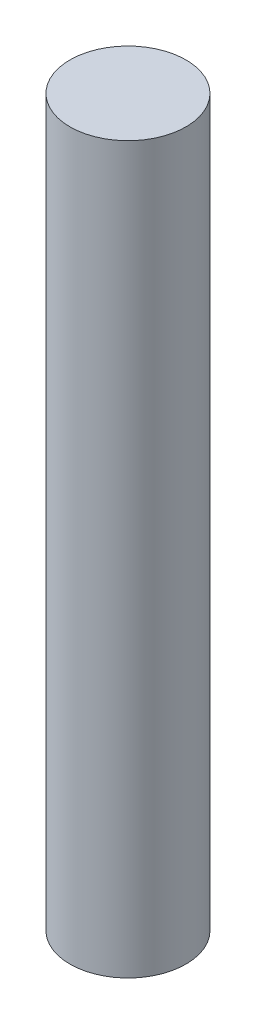
SolidWorks part; units mm, degrees
material "Q235"
ref_plane "Front Plane" through (0, 0, 0) normal (0, 0, 1) x (1, 0, 0)
ref_plane "Top Plane" through (0, 0, 0) normal (0, 1, 0) x (1, 0, 0)
ref_plane "Right Plane" through (0, 0, 0) normal (1, 0, 0) x (0, 0, -1)
sketch "Sketch1" plane through (0, 0, 0) normal (0, 1, 0) x (1, 0, 0)
  circle A0 centre (0, 0) radius 8
extrude "Boss-Extrude1" add sketch "Sketch1" along normal blind 100
